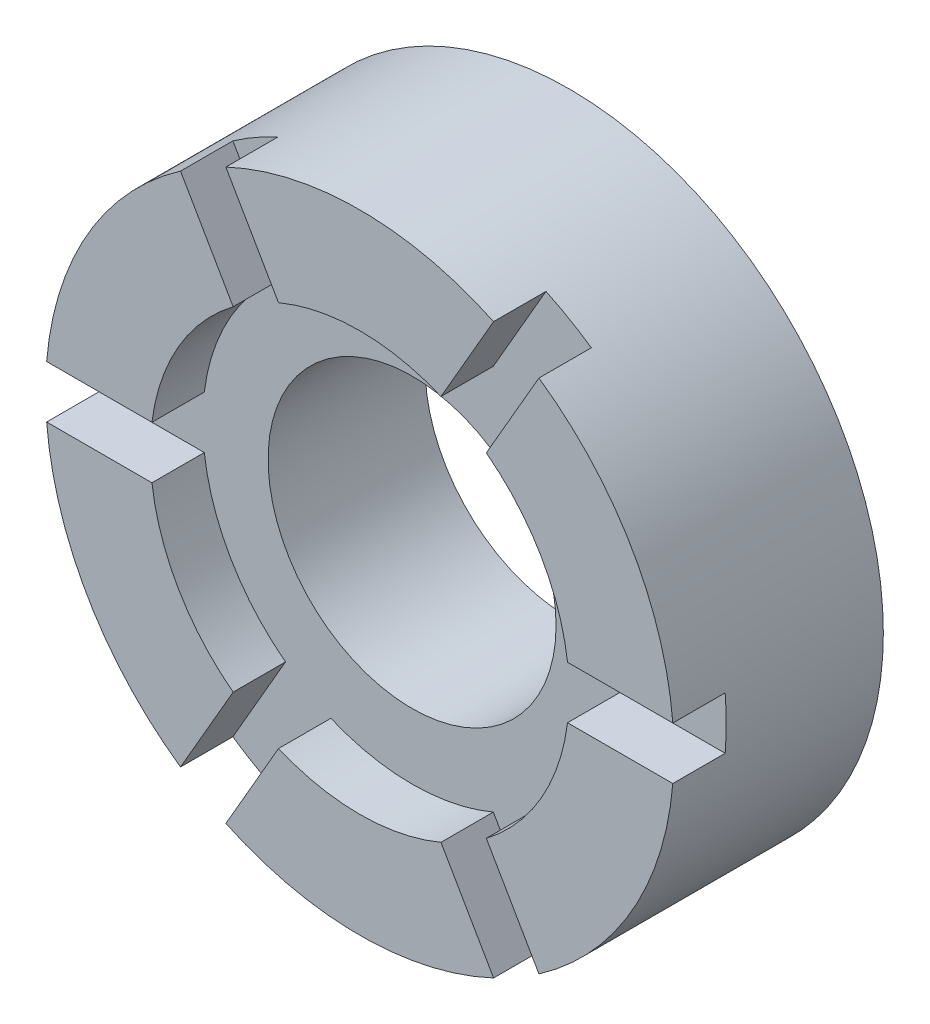
from build123d import *

# Parameters (mm, degrees)
SKETCH_1_R               = 60
EXTRUDE_1_DEPTH          = 40
SKETCH_2_R               = 40
CUT_EXTRUDE_1_DEPTH      = 10
CUT_EXTRUDE_2_REACH      = 92
SKETCH_3_R               = 27.5
SKETCH_4_W               = 150
SKETCH_4_H               = 10
CUT_EXTRUDE_3_DEPTH      = 10
PATTERN_CIRCULAR_1_COUNT = 3


with BuildPart() as part:
    # 草图1 → 凸台-拉伸1 (new body)
    with BuildSketch(Plane.XY):
        Circle(SKETCH_1_R)
    extrude(amount=EXTRUDE_1_DEPTH)

    # 草图2 → 切除-拉伸1 (cut)
    with BuildSketch(Plane.XY.offset(40)):
        Circle(SKETCH_2_R)
    extrude(amount=-CUT_EXTRUDE_1_DEPTH, mode=Mode.SUBTRACT)

    # 草图3 → 切除-拉伸2 (cut, up to next)
    with BuildSketch(Plane.XY.offset(30), mode=Mode.PRIVATE) as cut_extrude_2_sk1:
        Circle(SKETCH_3_R)
    cut_extrude_2_tool1 = extrude(cut_extrude_2_sk1.sketch, amount=-CUT_EXTRUDE_2_REACH, mode=Mode.PRIVATE) & part.part
    add(cut_extrude_2_tool1.solids().sort_by_distance((0, 0, 30))[0], mode=Mode.SUBTRACT)

    # 草图4 → 切除-拉伸3 (cut)
    with BuildSketch(Plane.XY.offset(30)):
        Rectangle(SKETCH_4_W, SKETCH_4_H)
    cut_extrude_3 = extrude(amount=CUT_EXTRUDE_3_DEPTH, mode=Mode.SUBTRACT)

    # 阵列(圆周)1: 切除-拉伸3 ×3 about axis
    pattern_circular_1_axis = Axis((0, 0, 0), (0, 0, 1))
    for i in range(1, PATTERN_CIRCULAR_1_COUNT):
        add(cut_extrude_3.rotate(pattern_circular_1_axis, i * 360 / PATTERN_CIRCULAR_1_COUNT), mode=Mode.SUBTRACT)


solid = part.part
